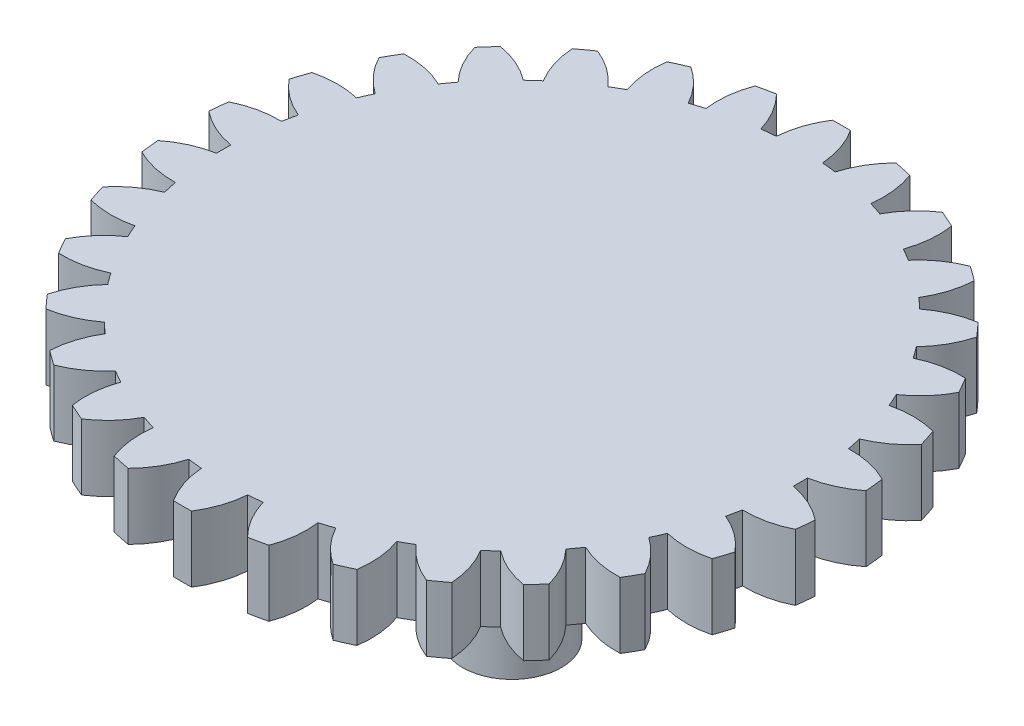
from build123d import *

# Parameters (mm, degrees)
SKETCH1_R           = 30
BOSS_EXTRUDE1_DEPTH = 100
SKETCH2_R           = 50
BOSS_EXTRUDE2_DEPTH = 30
BOSS_EXTRUDE3_DEPTH = 40


with BuildPart() as part:
    # Sketch1 → Boss-Extrude1 (new body)
    with BuildSketch(Plane(origin=(0, 0, 0), x_dir=(1, 0, 0), z_dir=(0, 1, 0))):
        with Locations(Location((0, 0, 0), (0, 0, 270))):
            Circle(SKETCH1_R)
    extrude(amount=BOSS_EXTRUDE1_DEPTH)

    # Sketch2 → Boss-Extrude2 (add)
    with BuildSketch(Plane(origin=(0, 100, 0), x_dir=(1, 0, 0), z_dir=(0, 1, 0))):
        with Locations(Location((0, 0, 0), (0, 0, 270))):
            Circle(SKETCH2_R)
    extrude(amount=BOSS_EXTRUDE2_DEPTH)


with BuildPart() as body_2:
    # Sketch3 → Boss-Extrude3 (new body)
    with BuildSketch(Plane(origin=(0, 130, 0), x_dir=(1, 0, 0), z_dir=(0, 1, 0))):
        with BuildLine():
            ThreePointArc((5.499480054, 199.924375), (0, 200), (-5.499480054, 199.924375))
            ThreePointArc((-5.499480054, 199.924375), (-11.329745737, 187.70874319), (-14, 174.439101121))
            ThreePointArc((-14, 174.439101121), (-18.292481072, 174.041331689), (-22.573862049, 173.537951907))
            ThreePointArc((-22.573862049, 173.537951907), (-27.944678568, 185.962443381), (-36.187311622, 196.698953931))
            ThreePointArc((-36.187311622, 196.698953931), (-41.582338164, 195.629520147), (-46.945918062, 194.412141538))
            ThreePointArc((-46.945918062, 194.412141538), (-50.109005787, 181.251270195), (-49.961994869, 167.716424564))
            ThreePointArc((-49.961994869, 167.716424564), (-54.077974016, 166.434890352), (-58.161138004, 165.052361468))
            ThreePointArc((-58.161138004, 165.052361468), (-65.997786327, 176.088692449), (-76.292544134, 184.876844709))
            ThreePointArc((-76.292544134, 184.876844709), (-81.347328615, 182.709091529), (-86.340594179, 180.403164598))
            ThreePointArc((-86.340594179, 180.403164598), (-86.698261835, 166.872246953), (-83.740410818, 153.663735462))
            ThreePointArc((-83.740410818, 153.663735462), (-87.5, 151.554445662), (-91.206493141, 149.353190823))
            ThreePointArc((-91.206493141, 149.353190823), (-101.16647413, 158.51902069), (-113.063426375, 164.974730236))
            ThreePointArc((-113.063426375, 164.974730236), (-117.557050458, 161.803398875), (-121.961772022, 158.509703694))
            ThreePointArc((-121.961772022, 158.509703694), (-119.498387816, 145.200105777), (-113.858968983, 132.895203759))
            ThreePointArc((-113.858968983, 132.895203759), (-117.097856113, 130.050344459), (-120.26568687, 127.126569063))
            ThreePointArc((-120.26568687, 127.126569063), (-131.913701564, 134.021307068), (-144.892894345, 137.862428414))
            ThreePointArc((-144.892894345, 137.862428414), (-148.628965095, 133.826121272), (-152.252635191, 129.688608125))
            ThreePointArc((-152.252635191, 129.688608125), (-147.075860833, 117.182023231), (-139.001343848, 106.318513949))
            ThreePointArc((-139.001343848, 106.318513949), (-141.577974016, 102.862419151), (-144.068692984, 99.343906214))
            ThreePointArc((-144.068692984, 99.343906214), (-156.895667246, 103.666219221), (-170.389847559, 104.724876934))
            ThreePointArc((-170.389847559, 104.724876934), (-173.205080757, 100), (-175.889327613, 95.199498066))
            ThreePointArc((-175.889327613, 95.199498066), (-168.225412983, 84.042523968), (-158.068692984, 75.095194908))
            ThreePointArc((-158.068692984, 75.095194908), (-159.870455087, 71.178912538), (-161.575205897, 67.219437958))
            ThreePointArc((-161.575205897, 67.219437958), (-175.020539402, 68.780420149), (-188.439946813, 67.010345806))
            ThreePointArc((-188.439946813, 67.010345806), (-190.211303259, 61.803398875), (-191.838812407, 56.549713124))
            ThreePointArc((-191.838812407, 56.549713124), (-182.022707351, 47.229963127), (-170.227681739, 40.589855502))
            ThreePointArc((-170.227681739, 40.589855502), (-171.175830128, 36.384545893), (-172.020106988, 32.157157709))
            ThreePointArc((-172.020106988, 32.157157709), (-185.496174143, 30.888586672), (-198.254316157, 26.367141015))
            ThreePointArc((-198.254316157, 26.367141015), (-198.904379074, 20.905692654), (-199.404020554, 15.428434362))
            ThreePointArc((-199.404020554, 15.428434362), (-187.864735965, 8.353226263), (-174.946903959, 4.310544639))
            ThreePointArc((-174.946903959, 4.310544639), (-175, 0), (-174.946903959, -4.310544639))
            ThreePointArc((-174.946903959, -4.310544639), (-187.864735965, -8.353226263), (-199.404020554, -15.428434362))
            ThreePointArc((-199.404020554, -15.428434362), (-198.904379074, -20.905692654), (-198.254316157, -26.367141015))
            ThreePointArc((-198.254316157, -26.367141015), (-185.496174143, -30.888586672), (-172.020106988, -32.157157709))
            ThreePointArc((-172.020106988, -32.157157709), (-171.175830128, -36.384545893), (-170.227681739, -40.589855502))
            ThreePointArc((-170.227681739, -40.589855502), (-182.022707351, -47.229963127), (-191.838812407, -56.549713124))
            ThreePointArc((-191.838812407, -56.549713124), (-190.211303259, -61.803398875), (-188.439946813, -67.010345806))
            ThreePointArc((-188.439946813, -67.010345806), (-175.020539402, -68.780420149), (-161.575205897, -67.219437958))
            ThreePointArc((-161.575205897, -67.219437958), (-159.870455087, -71.178912538), (-158.068692984, -75.095194908))
            ThreePointArc((-158.068692984, -75.095194908), (-168.225412983, -84.042523968), (-175.889327613, -95.199498066))
            ThreePointArc((-175.889327613, -95.199498066), (-173.205080757, -100), (-170.389847559, -104.724876934))
            ThreePointArc((-170.389847559, -104.724876934), (-156.895667246, -103.666219221), (-144.068692984, -99.343906214))
            ThreePointArc((-144.068692984, -99.343906214), (-141.577974016, -102.862419151), (-139.001343848, -106.318513949))
            ThreePointArc((-139.001343848, -106.318513949), (-147.075860833, -117.182023231), (-152.252635191, -129.688608125))
            ThreePointArc((-152.252635191, -129.688608125), (-148.628965095, -133.826121272), (-144.892894345, -137.862428414))
            ThreePointArc((-144.892894345, -137.862428414), (-131.913701564, -134.021307068), (-120.26568687, -127.126569063))
            ThreePointArc((-120.26568687, -127.126569063), (-117.097856113, -130.050344459), (-113.858968983, -132.895203759))
            ThreePointArc((-113.858968983, -132.895203759), (-119.498387816, -145.200105777), (-121.961772022, -158.509703694))
            ThreePointArc((-121.961772022, -158.509703694), (-117.557050458, -161.803398875), (-113.063426375, -164.974730236))
            ThreePointArc((-113.063426375, -164.974730236), (-101.16647413, -158.51902069), (-91.206493141, -149.353190823))
            ThreePointArc((-91.206493141, -149.353190823), (-87.5, -151.554445662), (-83.740410818, -153.663735462))
            ThreePointArc((-83.740410818, -153.663735462), (-86.698261835, -166.872246953), (-86.340594179, -180.403164598))
            ThreePointArc((-86.340594179, -180.403164598), (-81.347328615, -182.709091529), (-76.292544134, -184.876844709))
            ThreePointArc((-76.292544134, -184.876844709), (-65.997786327, -176.088692449), (-58.161138004, -165.052361468))
            ThreePointArc((-58.161138004, -165.052361468), (-54.077974016, -166.434890352), (-49.961994869, -167.716424564))
            ThreePointArc((-49.961994869, -167.716424564), (-50.109005787, -181.251270195), (-46.945918062, -194.412141538))
            ThreePointArc((-46.945918062, -194.412141538), (-41.582338164, -195.629520147), (-36.187311622, -196.698953931))
            ThreePointArc((-36.187311622, -196.698953931), (-27.944678568, -185.962443381), (-22.573862049, -173.537951907))
            ThreePointArc((-22.573862049, -173.537951907), (-18.292481072, -174.041331689), (-14, -174.439101121))
            ThreePointArc((-14, -174.439101121), (-11.329745737, -187.70874319), (-5.499480054, -199.924375))
            ThreePointArc((-5.499480054, -199.924375), (0, -200), (5.499480054, -199.924375))
            ThreePointArc((5.499480054, -199.924375), (11.329745737, -187.70874319), (14, -174.439101121))
            ThreePointArc((14, -174.439101121), (18.292481072, -174.041331689), (22.573862049, -173.537951907))
            ThreePointArc((22.573862049, -173.537951907), (27.944678568, -185.962443381), (36.187311622, -196.698953931))
            ThreePointArc((36.187311622, -196.698953931), (41.582338164, -195.629520147), (46.945918062, -194.412141538))
            ThreePointArc((46.945918062, -194.412141538), (50.109005787, -181.251270195), (49.961994869, -167.716424564))
            ThreePointArc((49.961994869, -167.716424564), (54.077974016, -166.434890352), (58.161138004, -165.052361468))
            ThreePointArc((58.161138004, -165.052361468), (65.997786327, -176.088692449), (76.292544134, -184.876844709))
            ThreePointArc((76.292544134, -184.876844709), (81.347328615, -182.709091529), (86.340594179, -180.403164598))
            ThreePointArc((86.340594179, -180.403164598), (86.698261835, -166.872246953), (83.740410818, -153.663735462))
            ThreePointArc((83.740410818, -153.663735462), (87.5, -151.554445662), (91.206493141, -149.353190823))
            ThreePointArc((91.206493141, -149.353190823), (101.16647413, -158.51902069), (113.063426375, -164.974730236))
            ThreePointArc((113.063426375, -164.974730236), (117.557050458, -161.803398875), (121.961772022, -158.509703694))
            ThreePointArc((121.961772022, -158.509703694), (119.498387816, -145.200105777), (113.858968983, -132.895203759))
            ThreePointArc((113.858968983, -132.895203759), (117.097856113, -130.050344459), (120.26568687, -127.126569063))
            ThreePointArc((120.26568687, -127.126569063), (131.913701564, -134.021307068), (144.892894345, -137.862428414))
            ThreePointArc((144.892894345, -137.862428414), (148.628965095, -133.826121272), (152.252635191, -129.688608125))
            ThreePointArc((152.252635191, -129.688608125), (147.075860833, -117.182023231), (139.001343848, -106.318513949))
            ThreePointArc((139.001343848, -106.318513949), (141.577974016, -102.862419151), (144.068692984, -99.343906214))
            ThreePointArc((144.068692984, -99.343906214), (156.895667246, -103.666219221), (170.389847559, -104.724876934))
            ThreePointArc((170.389847559, -104.724876934), (173.205080757, -100), (175.889327613, -95.199498066))
            ThreePointArc((175.889327613, -95.199498066), (168.225412983, -84.042523968), (158.068692984, -75.095194908))
            ThreePointArc((158.068692984, -75.095194908), (159.870455087, -71.178912538), (161.575205897, -67.219437958))
            ThreePointArc((161.575205897, -67.219437958), (175.020539402, -68.780420149), (188.439946813, -67.010345806))
            ThreePointArc((188.439946813, -67.010345806), (190.211303259, -61.803398875), (191.838812407, -56.549713124))
            ThreePointArc((191.838812407, -56.549713124), (182.022707351, -47.229963127), (170.227681739, -40.589855502))
            ThreePointArc((170.227681739, -40.589855502), (171.175830128, -36.384545893), (172.020106988, -32.157157709))
            ThreePointArc((172.020106988, -32.157157709), (185.496174143, -30.888586672), (198.254316157, -26.367141015))
            ThreePointArc((198.254316157, -26.367141015), (198.904379074, -20.905692654), (199.404020554, -15.428434362))
            ThreePointArc((199.404020554, -15.428434362), (187.864735965, -8.353226263), (174.946903959, -4.310544639))
            ThreePointArc((174.946903959, -4.310544639), (175, 0), (174.946903959, 4.310544639))
            ThreePointArc((174.946903959, 4.310544639), (187.864735965, 8.353226263), (199.404020554, 15.428434362))
            ThreePointArc((199.404020554, 15.428434362), (198.904379074, 20.905692654), (198.254316157, 26.367141015))
            ThreePointArc((198.254316157, 26.367141015), (185.496174143, 30.888586672), (172.020106988, 32.157157709))
            ThreePointArc((172.020106988, 32.157157709), (171.175830128, 36.384545893), (170.227681739, 40.589855502))
            ThreePointArc((170.227681739, 40.589855502), (182.022707351, 47.229963127), (191.838812407, 56.549713124))
            ThreePointArc((191.838812407, 56.549713124), (190.211303259, 61.803398875), (188.439946813, 67.010345806))
            ThreePointArc((188.439946813, 67.010345806), (175.020539402, 68.780420149), (161.575205897, 67.219437958))
            ThreePointArc((161.575205897, 67.219437958), (159.870455087, 71.178912538), (158.068692984, 75.095194908))
            ThreePointArc((158.068692984, 75.095194908), (168.225412983, 84.042523968), (175.889327613, 95.199498066))
            ThreePointArc((175.889327613, 95.199498066), (173.205080757, 100), (170.389847559, 104.724876934))
            ThreePointArc((170.389847559, 104.724876934), (156.895667246, 103.666219221), (144.068692984, 99.343906214))
            ThreePointArc((144.068692984, 99.343906214), (141.577974016, 102.862419151), (139.001343848, 106.318513949))
            ThreePointArc((139.001343848, 106.318513949), (147.075860833, 117.182023231), (152.252635191, 129.688608125))
            ThreePointArc((152.252635191, 129.688608125), (148.628965095, 133.826121272), (144.892894345, 137.862428414))
            ThreePointArc((144.892894345, 137.862428414), (131.913701564, 134.021307068), (120.26568687, 127.126569063))
            ThreePointArc((120.26568687, 127.126569063), (117.097856113, 130.050344459), (113.858968983, 132.895203759))
            ThreePointArc((113.858968983, 132.895203759), (119.498387816, 145.200105777), (121.961772022, 158.509703694))
            ThreePointArc((121.961772022, 158.509703694), (117.557050458, 161.803398875), (113.063426375, 164.974730236))
            ThreePointArc((113.063426375, 164.974730236), (101.16647413, 158.51902069), (91.206493141, 149.353190823))
            ThreePointArc((91.206493141, 149.353190823), (87.5, 151.554445662), (83.740410818, 153.663735462))
            ThreePointArc((83.740410818, 153.663735462), (86.698261835, 166.872246953), (86.340594179, 180.403164598))
            ThreePointArc((86.340594179, 180.403164598), (81.347328615, 182.709091529), (76.292544134, 184.876844709))
            ThreePointArc((76.292544134, 184.876844709), (65.997786327, 176.088692449), (58.161138004, 165.052361468))
            ThreePointArc((58.161138004, 165.052361468), (54.077974016, 166.434890352), (49.961994869, 167.716424564))
            ThreePointArc((49.961994869, 167.716424564), (50.109005787, 181.251270195), (46.945918062, 194.412141538))
            ThreePointArc((46.945918062, 194.412141538), (41.582338164, 195.629520147), (36.187311622, 196.698953931))
            ThreePointArc((36.187311622, 196.698953931), (27.944678568, 185.962443381), (22.573862049, 173.537951907))
            ThreePointArc((22.573862049, 173.537951907), (18.292481072, 174.041331689), (14, 174.439101121))
            ThreePointArc((14, 174.439101121), (11.329745737, 187.70874319), (5.499480054, 199.924375))
        make_face()
    extrude(amount=BOSS_EXTRUDE3_DEPTH)


solid = Compound([part.part, body_2.part])
